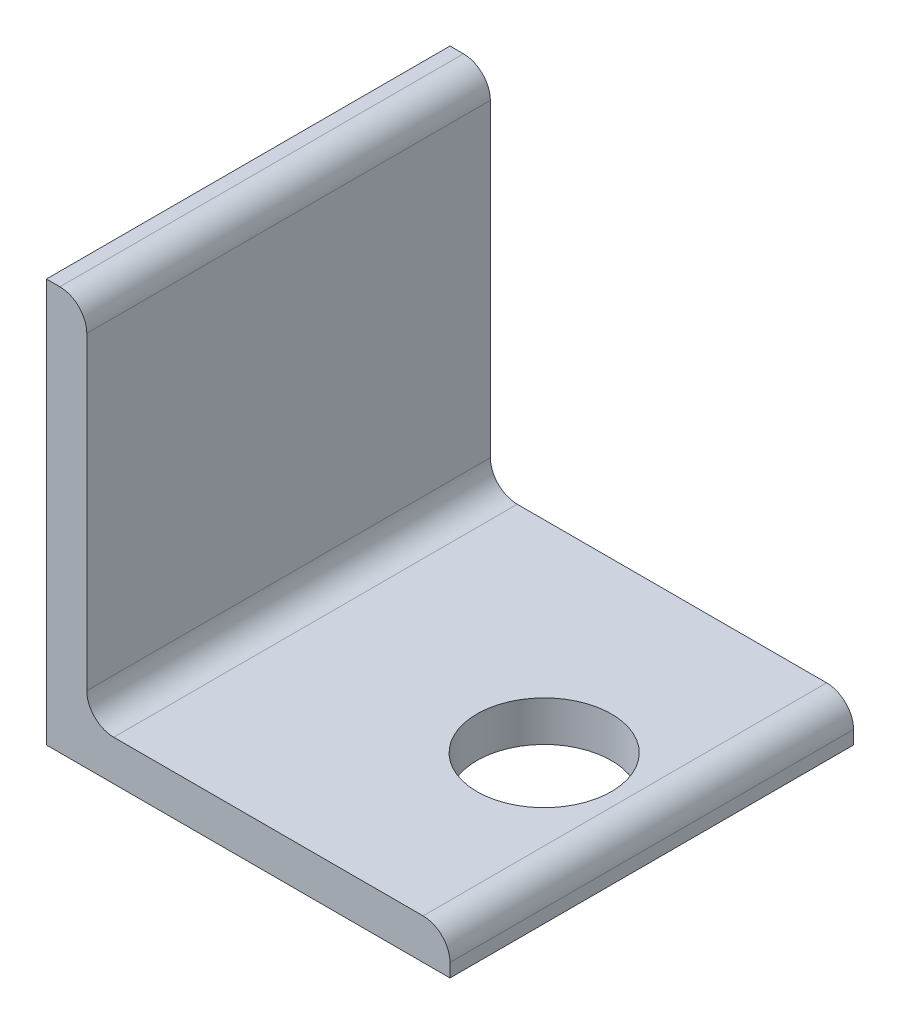
from build123d import *

# Parameters (mm, degrees)
BOSS_EXTRUDE1_DEPTH = 30
SKETCH3_R           = 5
CUT_EXTRUDE1_DEPTH  = 3


with BuildPart() as part:
    # Sketch2 → Boss-Extrude1 (new body)
    with BuildSketch(Plane.XY):
        with BuildLine():
            Line((0, 0), (0, 30))
            Line((0, 30), (1, 30))
            ThreePointArc((1, 30), (2.414213562, 29.414213562), (3, 28))
            Line((3, 28), (3, 5))
            ThreePointArc((3, 5), (3.585786438, 3.585786438), (5, 3))
            Line((5, 3), (28, 3))
            ThreePointArc((28, 3), (29.414213562, 2.414213562), (30, 1))
            Line((30, 1), (30, 0))
            Line((30, 0), (0, 0))
        make_face()
    extrude(amount=BOSS_EXTRUDE1_DEPTH)

    # Sketch3 → Cut-Extrude1 (cut)
    with BuildSketch(Plane(origin=(0, 3, 0), x_dir=(1, 0, 0), z_dir=(0, 1, 0))):
        with Locations(Location((22, -15, 0), (0, 0, 270))):
            Circle(SKETCH3_R)
    extrude(amount=-CUT_EXTRUDE1_DEPTH, mode=Mode.SUBTRACT)


solid = part.part
